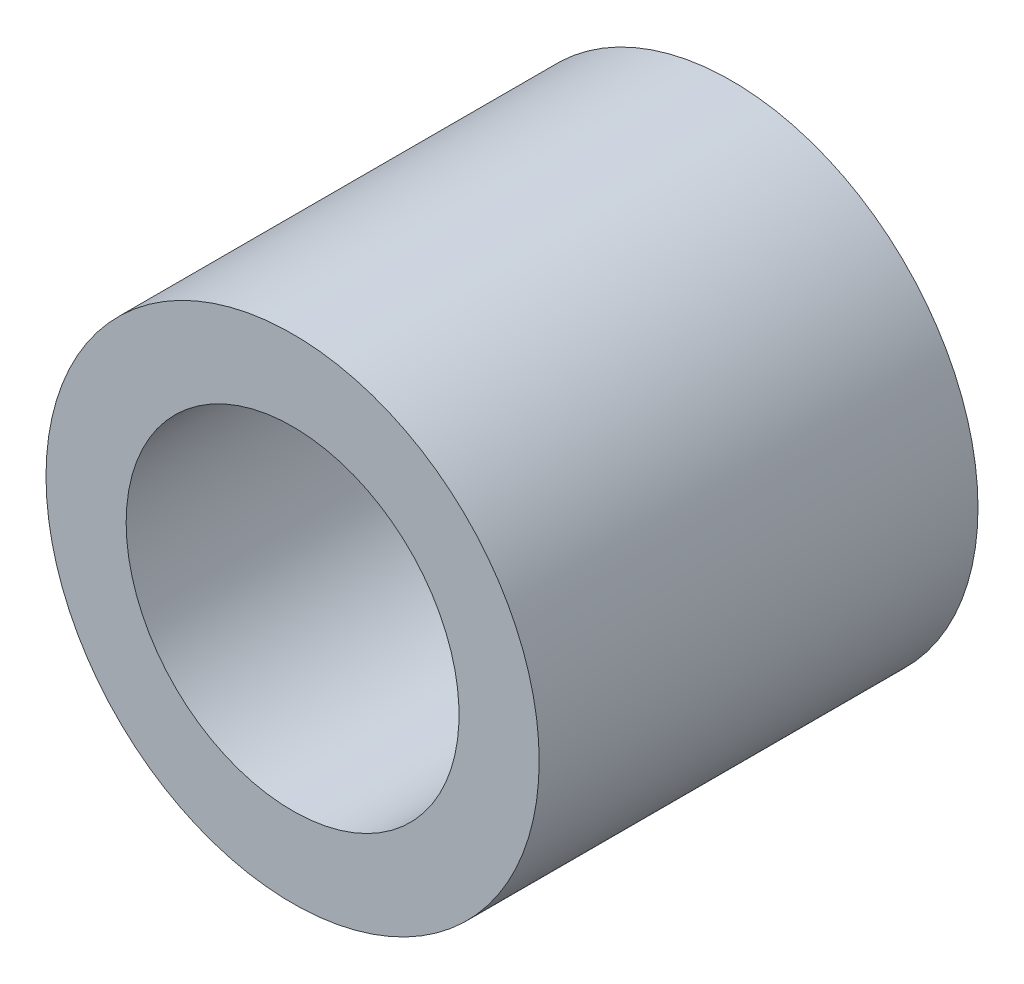
SolidWorks part; units mm, degrees
ref_plane "Front Plane" through (0, 0, 0) normal (0, 0, 1) x (1, 0, 0)
ref_plane "Top Plane" through (0, 0, 0) normal (0, 1, 0) x (1, 0, 0)
ref_plane "Right Plane" through (0, 0, 0) normal (1, 0, 0) x (0, 0, -1)
sketch "Sketch1" plane through (0, 0, 0) normal (0, 0, 1) x (1, 0, 0)
  circle A0 centre (10, -61.7532) radius 4.05
  circle A1 centre (10, -61.7532) radius 6
  dimension "D1" = 8.1
  dimension "D2" = 12
extrude "Boss-Extrude1" add sketch "Sketch1" along normal up to surface (10.6769 mm away)
